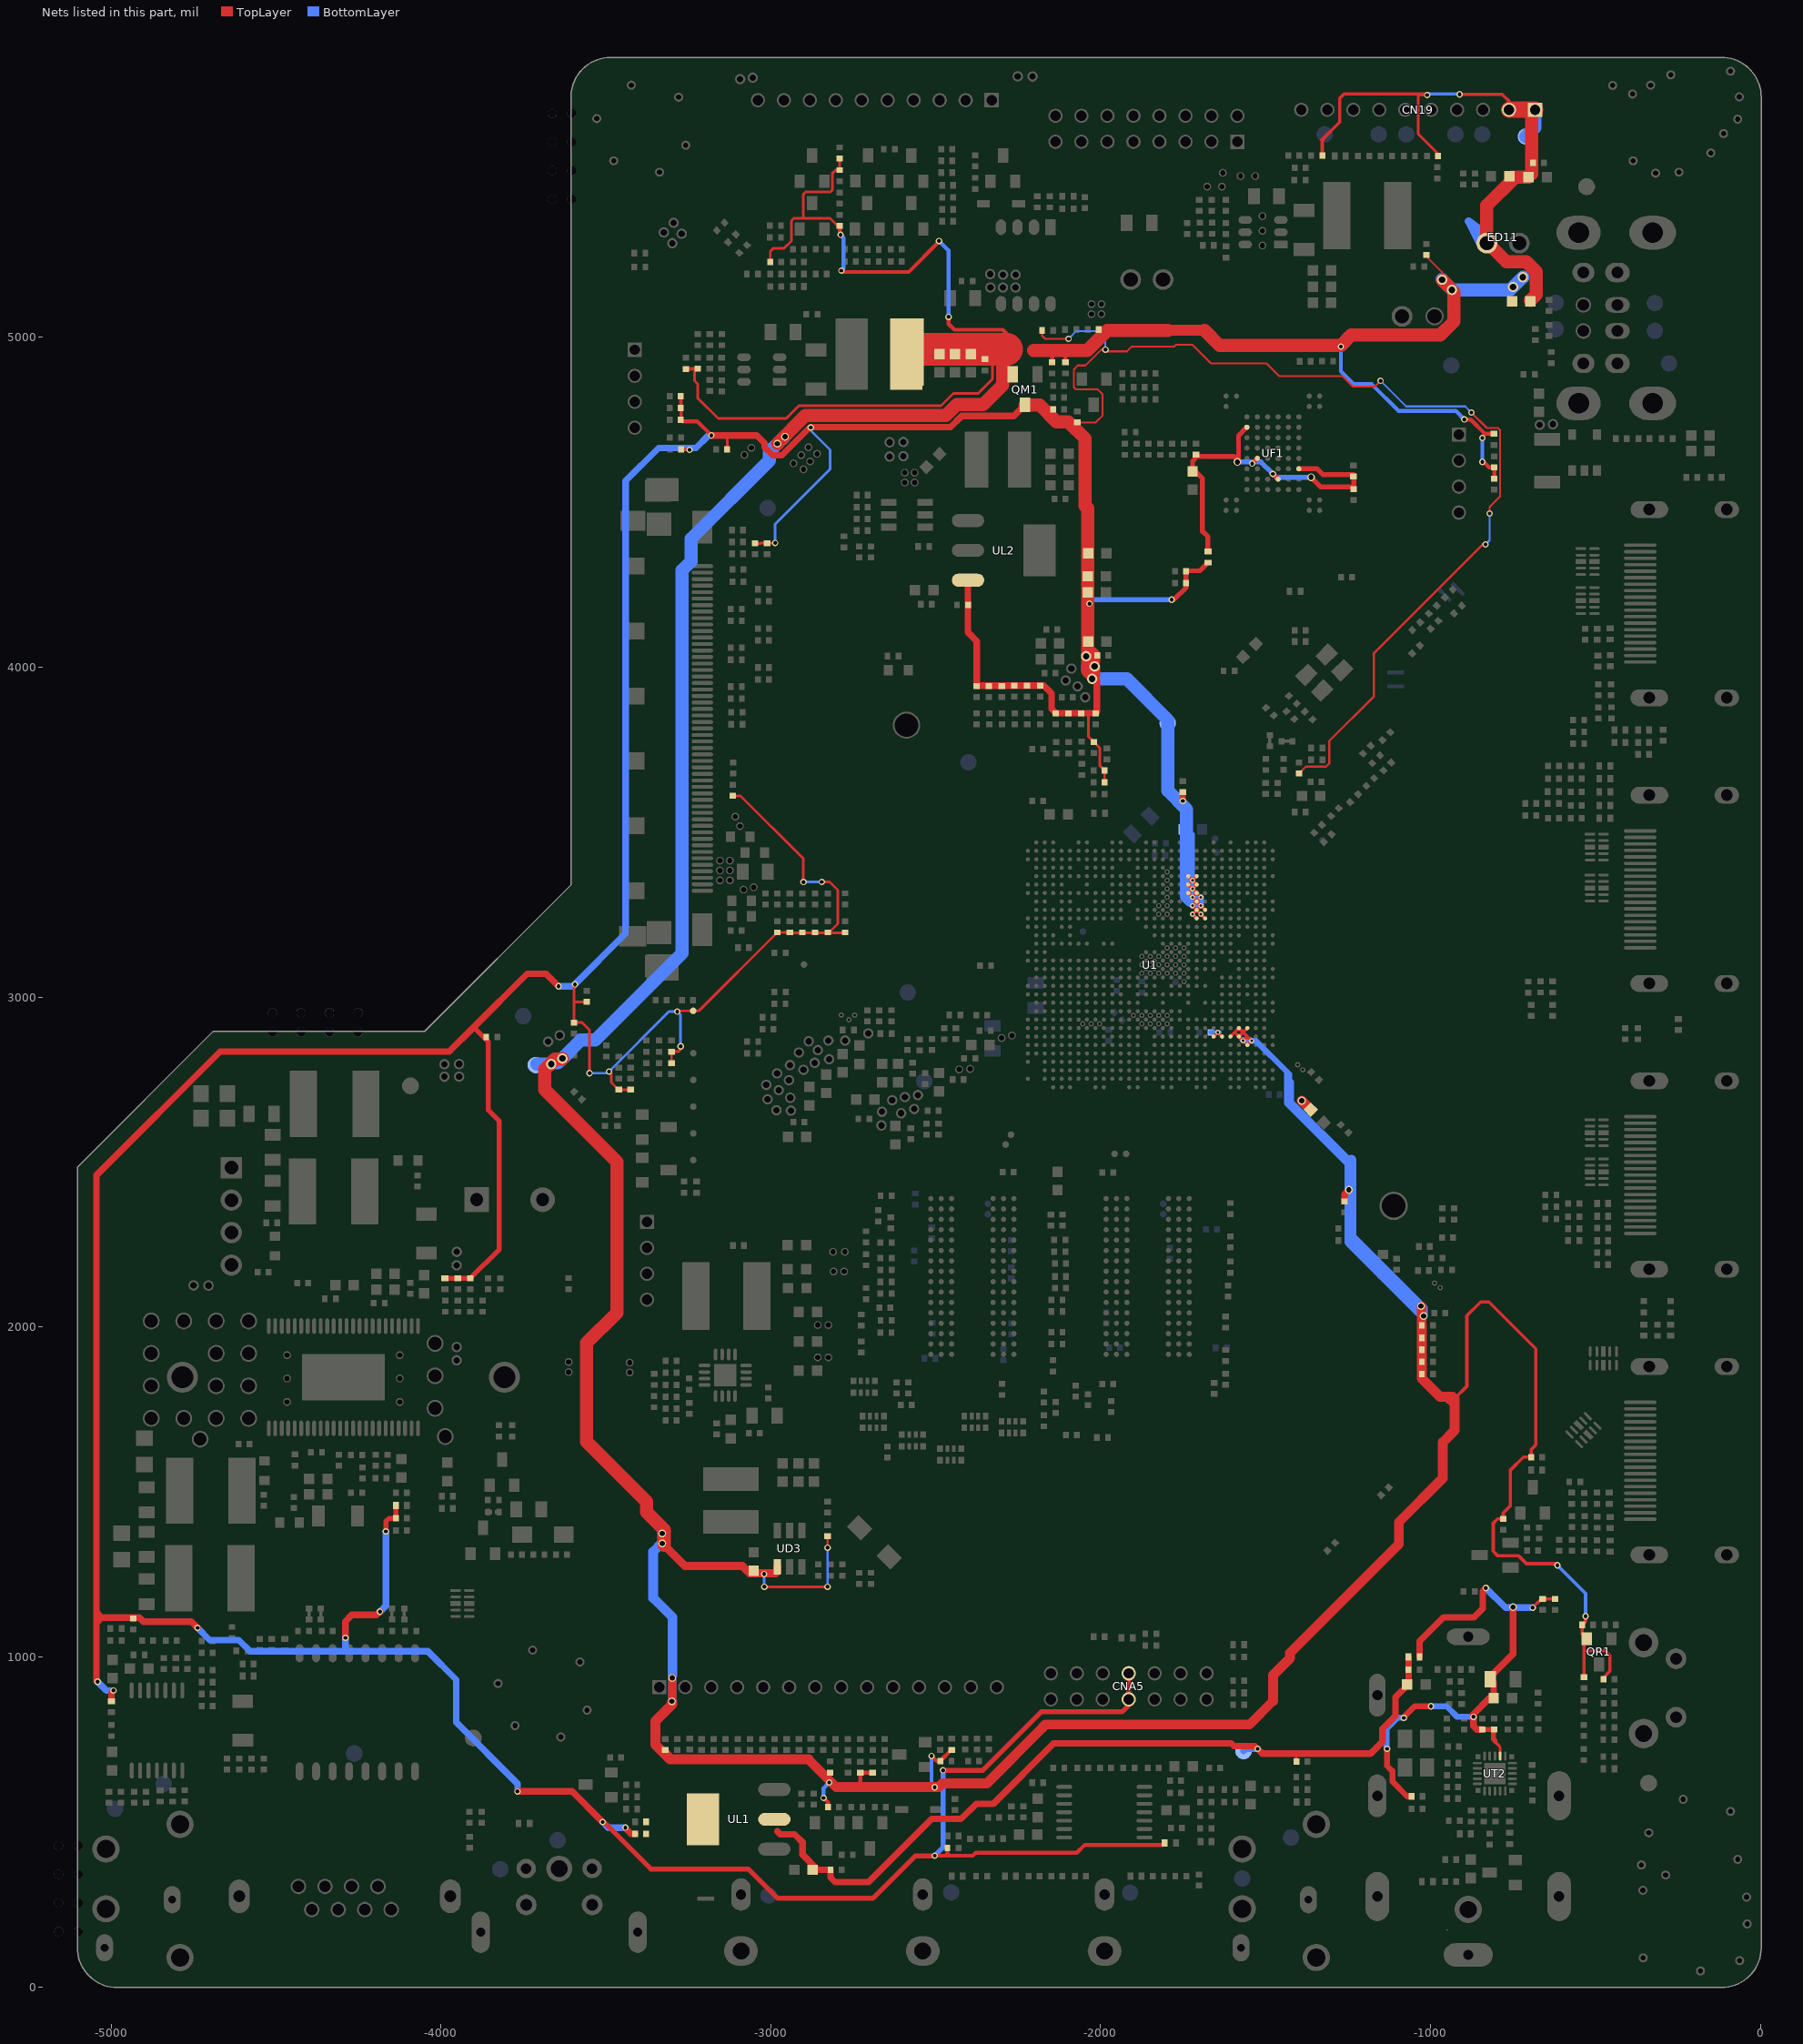
[diagram p0: the nets of this part, all layers, seen from the top]
# Altium PCB MISC86290.PcbDoc (part 9 of 31)
Units mil, origin at the board's own origin, x right, y up, seen from the top; angles counter-clockwise.
Board outline 5104.71 x 5851.49 mil, 2 copper layers (TopLayer, BottomLayer), stack 61.855 mil thick; 1026 components, 667 nets, 4280 pads, 2294 vias.

## Via types
v1: diameter 19.68, hole 11.81, TopLayer to BottomLayer, tented both sides, 1189 vias
v2: diameter 19.68/19.68 (per signal layer), hole 11.81, TopLayer to BottomLayer, tented both sides, 366 vias
v3: diameter 15.75, hole 7.87, TopLayer to BottomLayer, tented both sides, 348 vias
v4: diameter 23.62, hole 15.75, TopLayer to BottomLayer, tented both sides, 309 vias
v5: diameter 15.75/15.75 (per signal layer), hole 7.87, TopLayer to BottomLayer, tented both sides, 59 vias
v6: diameter 24/24 (per signal layer), hole 16, TopLayer to BottomLayer, tented both sides, 23 vias

## Nets (pads, with @x,y where several pads share a name; then routed paths per layer and width w, separated by ;. In a path a pad name is that pad's centre, name@x,y a point inside that pad or via, vN(x,y) a via of type N, cw(c..) or ccw(c..) an arc to the next point about the centre after c; other vN are vias at no path point) (continued)
3V3_M: 3V3_M.1 3V3_N.1 C16.2 C17.1 C18.1 C19.2 C20.1 C21.2 C22.1 C23.1 C240.2 CL55.2 CM2.2 CM3.2 CNA5.7 CNA5.8 LA10.1 LA12.1 LF1.2 LO2.2 LO3.2 pad.VIA5@-1696.18,3251.57 pad.VIA5@-1696.18,3277.17 pad.VIA5@-1696.18,3302.76 pad.VIA5@-1721.77,3251.57 pad.VIA5@-1721.77,3277.17 pad.VIA5@-1721.77,3302.76 pad.VIA5@-1721.77,3328.35 pad.VIA5@-1721.77,3353.94 pad.VIA5@-2018.5,4002.5 pad.VIA5@-2026,3965 pad.VIA5@-2044,4033.5 QM1.D R4.2 R5.2 R6.2 R7.2 R12.2 R13.2 R14.2 R15.2 R16.2 R17.2 R18.2 R19.2 R30.2 R31.2 R122.2 R124.2 R143.2 R144.2 R145.2 R171.2 R206.2 R207.2 RA5.1 RA34.1 RD24.2 RG6.2 RG16.2 RO46.2 RO47.2 RP5.2 RT7.2 RT40.1 RU5.1 RW8.1 RW9.1 RW251.2 RW405.2 RW406.2 RW407.2 RW408.2 RW409.2 RW410.2 U1.AA9 U1.AA10 U1.AB9 U1.AB10 U1.AC10 U1.AD10 U1.AD11 U1.AE10 U1.AE11 U1.AF10 U1.AF11 UL2.3 | length 23311.8
  TopLayer w6: RP5.2@-2177.73,5024 RP5.2@-2177.73,5021 -2177.73,5005.25 -2167.98,4995.5 v1(-2097.5,4995.5) ; C17.1@-2071,4742.27 -2015.22,4742.27 -1994,4763.49 -1994,4827.5 -2008.73,4842.23 -2075.45,4842.23 -2081.5,4848.28 -2081.5,4903 -2069.5,4915 -2046,4915 -1998,4963 v1(-1985.5,4963) -1980.16,4957.66 -1920.61,4957.66 -1905.61,4972.66 -1777.22,4972.66 -1771.89,4977.99 -1722.49,4977.99 -1665.49,4920.99 -1497.05,4920.99 -1458.55,4882.5 -1267.05,4882.5 -1235.68,4851.13 -1168.87,4851.13 v1(-1151.5,4868.5) ; v1(-876,4772) -829.5,4725.5 -795.5,4725.5 -789.16,4719.16 -789.16,4518.29 -821,4486.45 v1(-821,4466)
  TopLayer w7: RT7.2@-1398.5,3678.27 -1377.93,3698.84 -1316.66,3698.84 -1307.5,3708 -1307.5,3776.08 -1171.77,3911.81 -1171.77,4042.92 -842.22,4372.47 v1(-833.25,4372.47)
  TopLayer w8: -3596.97,2985.47 RG16.2@-3557.76,2985.47 ; v1(-3594.16,3038.7) -3597,3035.86 R143.2@-3597,2922.73 -3572.12,2922.73 -3549.35,2899.97 v1(-3549.35,2769.45) v1@-3549.35,2765.16 ; v1(-3490.5,2774.5) -3483.5,2767.5 -3483.5,2741 -3461.77,2719.27 R145.2@-3425,2719.27 ; R207.2@-3301,2800.23 R206.2@-3301,2834.77 -3280.23,2834.77 -3273.5,2841.5 v1(-3273.5,2851) ; v1(-3283.5,2956) -3284,2956.5 -3284,2958.5 3V3_N.1@-3235.5,2958.5 -3218.27,2958.5 RW405.2@-2980.5,3196.27 RW406.2@-2942.5,3196.27 ; R30.2@-3272.77,4750.37 R31.2@-3272.77,4786.37 ; RD24.2@-3272.27,4660.5 -3247.62,4660.5 v1(-3246.62,4659.5) ; R30.2@-3270.77,4754.26 R31.2@-3270.77,4786.37 ; RG6.2@-3132.5,4661 -3132.5,4700 ; RW408.2@-3115,3610.27 -3092.07,3610.27 -2902,3420.2 -2902,3348 v1(-2901,3349) ; RW8.1@-3047.5,4375.73 -3032,4375.73 -3030.83,4376.9 v1(-2986.82,4376.9) ; RW406.2@-2942.5,3194.8 RW409.2@-2824.55,3194.8 ; v1(-2879,4726.5) v1@-2877.5,4728 ; v1(-2845.66,3349.34) -2821.34,3349.34 -2796.75,3324.75 -2796.75,3222.6 RW409.2@-2824.55,3194.8 ; RW407.2@-2776.47,3194.8 RW409.2@-2824.55,3194.8 ; -2041.73,3860.73 -2037,3856 -2037,3789.73 R17.2@-2021,3773.73 -2002.16,3754.89 -2002.16,3727.68 -2003,3726.84 -2003,3701.73 R19.2@-1988.27,3687 R7.2@-1988.27,3651
  TopLayer w10: RW407.2@-2776.47,3194.8 RW407.2@-2775,3196.27 ; -2472.46,397 -2464.73,404.73 ; RO46.2@-2464.73,421 -2464.73,404.73 ; -2457,397 -2464.73,404.73 ; -2236.07,3943.23 R14.2@-2223.75,3943.23 ; U1.AF11@-1734.57,3366.73 pad.VIA5@-1721.77,3353.94 ; U1.AA10@-1708.98,3238.78 pad.VIA5@-1721.77,3251.57 U1.AB10@-1708.98,3264.37 ; U1.AF10@-1708.98,3366.73 pad.VIA5@-1721.77,3353.94 ; U1.AA9@-1683.39,3238.78 pad.VIA5@-1696.18,3251.57 U1.AB10@-1708.98,3264.37 ; U1.AB9@-1683.39,3264.37 pad.VIA5@-1696.18,3277.17 ; pad.VIA5@-1721.77,3302.76 U1.AC10@-1708.98,3289.96 ; pad.VIA5@-1721.77,3302.76 U1.AD11@-1734.57,3315.55 pad.VIA5@-1721.77,3328.35 ; pad.VIA5@-1721.77,3302.76 U1.AD10@-1708.98,3315.55 ; pad.VIA5@-1721.77,3328.35 U1.AE10@-1708.98,3341.14 pad.VIA5@-1721.77,3353.94 ; pad.VIA5@-1721.77,3328.35 U1.AE11@-1734.57,3341.14 pad.VIA5@-1721.77,3353.94 ; pad.VIA5@-1721.77,3328.35 U1.AD10@-1708.98,3315.55 ; U1.AB10@-1708.98,3264.37 pad.VIA5@-1696.18,3277.17 ; U1.AB10@-1708.98,3264.37 pad.VIA5@-1721.77,3277.17 U1.AC10@-1708.98,3289.96 ; U1.AC10@-1708.98,3289.96 pad.VIA5@-1696.18,3277.17 ; U1.AC10@-1708.98,3289.96 pad.VIA5@-1696.18,3302.76 U1.AD10@-1708.98,3315.55
  TopLayer w12: R31.2@-3272.77,4786.37 R171.2@-3272.77,4822.37 ; R30.2@-3267.74,4745.34 -3222.84,4745.34 v1(-3180.5,4703) ; v1(-2503.25,397) -2472.46,397 -2457,397 -2387.21,397 -2378.21,406 -2072.37,406 -2048.37,430 -1811.73,430 LO2.2@-1805.74,436
  TopLayer w15: v1(-4167,1380) -4167,1410 -4157,1420 RA5.1@-4136.73,1420 LA12.1@-4136.73,1459 ; LA10.1@-3988,2147.73 -3911,2147.73 -3823,2235.73 -3823,2623.97 -3856.4,2657.37 -3856.4,2864.4 -3901.01,2909.01 ; v1@-3509.73,502.73 -3364,357 -3068,357 -2979,268 -2690.79,268 -2561.79,397 v1(-2503.25,397) ; v1(-2478,656) -2357.51,656 -2180.01,833.5 -1935.5,833.5 -1915,854 CNA5.8@-1915,871.26 CNA5.7@-1915,950 CNA5.7@-1915,962 ; v1(-1785,4205) -1778.18,4205 -1741.27,4241.92 C22.1@-1741.27,4255 C23.1@-1741.27,4291 ; C23.1@-1733.87,4292.37 -1699.89,4292.37 LF1.2@-1675,4317.26
  TopLayer w17: v1(-1751,3594.5) C18.1@-1751,3621.27
  TopLayer w20: v1(-5041,924.5) -5044.17,927.67 -5044.17,1104 ; LO3.2@-4999,870 -4999,892 v1(-4993,898) ; v1(-4738,1088) -4756.5,1106.5 -4902.07,1106.5 -4914.57,1119 -5029.17,1119 ; v1(-4289.5,1057.5) -4289.5,1107.5 -4270,1127 -4195,1127 v1(-4185,1137) ; v1(-3768,592) -3602.38,592 v1@-3513.11,502.73 ; v1@-3643.6,3032.9 -3681.7,3071 -3739.02,3071 -3901.01,2909.01 -3975.12,2834.89 -4669.65,2834.89 -5044.17,2460.37 -5044.17,1134 ; v1(-3441,482.28) -3440.91,480.66 -3423.4,463.15 RT40.1@-3412,463.15 ; v1(-3180.5,4703) -3042.64,4703 -3019.25,4679.6 -3019.25,4667.75 -2994.13,4642.63 -2966.28,4642.63 -2880.92,4728 -2877.5,4728 -2455.26,4728 -2421.48,4761.78 -2263.22,4761.78 -2229.28,4795.72 QM1.D@-2229,4795.72 ; UL2.3@-2402.27,4263.87 -2402.27,4105.43 -2375.86,4079.02 -2375.86,3955.06 ; R13.2@-2374.86,3944.23 R12.2@-2261.75,3944.23 R14.2@-2223.75,3944.23 -2172.06,3944.23 -2148.9,3921.07 -2148.9,3873.64 R4.2@-2136,3860.73 ; R4.2@-2134.32,3862.41 -2132.64,3860.73 R5.2@-2098,3860.73 -2041.73,3860.73 RU5.1@-2015,3860.73 -2011.45,3864.28 pad.VIA5@-2011.45,3960.45 ; -5044.17,1104 -5029.17,1119 ; -5044.17,1104 -5044.17,1134 ; -5044.17,1134 -5029.17,1119
  TopLayer w40: QM1.D@-2229,4795.72 -2185.72,4795.72 -2134,4744 -2098,4744 -2046.84,4692.84 -2046.84,4488.84 -2039.83,4481.83 CM3.2@-2039.83,4275.9 -2039.83,4205.9 -2039.83,4055.06 ; pad.VIA5@-2021.45,4002.5 -2021.45,3975.55 -2024,3973 -2039.83,3988.83 -2039.83,4033.5 -2039.83,4055.06 ; -2021.45,4021.5 -2021.45,4035.5 -2021.45,4036.68 -2039.83,4055.06
  BottomLayer w6: v1(-2097.5,4995.5) -2073.5,5019.5 -2005,5019.5 -1985.84,5000.34 -1985.84,4963.34 v1(-1985.5,4963) ; v1(-1151.5,4868.5) -1074,4791 -895,4791 v1(-876,4772) ; v1(-833.25,4372.47) -821,4384.72 v1(-821,4466)
  BottomLayer w8: v1(-3594.16,3038.7) v1@-3591.96,3036.5 ; v1(-3549.35,2769.45) -3495.55,2769.45 v1(-3490.5,2774.5) -3309,2956 v1(-3283.5,2956) -3273.5,2946 v1(-3273.5,2851) ; v1(-3246.62,4659.5) v1@-3244,4659.5 ; v1@-2985.6,4376.9 v1(-2986.82,4376.9) -2986.82,4433.71 -2820,4600.53 -2820,4658.87 -2880.92,4719.79 -2880.92,4724.59 v1(-2879,4726.5) ; v1(-2901,3349) -2900.66,3349.34 v1(-2845.66,3349.34)
  BottomLayer w12: pad.VIA5@-1721.77,3328.35 -1703.31,3309.88 ; -1704.64,3308.55 -1703.31,3309.88 ; pad.VIA5@-1696.18,3302.76 -1703.31,3309.88
  BottomLayer w15: v1(-2503.25,397) -2477.91,422.34 v1@-2477.91,652.66 ; v1(-2034,4192.7) -2021.7,4205 -1985,4205 ; -2006,4205 -1985,4205 ; v1(-1785,4205) -1985,4205 ; pad.VIA5@-1722.02,3310.05 -1722.02,3494 ; pad.VIA5@-1721.77,3277.17 -1721.77,3287.58 pad.VIA5@-1721.77,3302.76 -1721.77,3308.55 -1708.22,3308.55 -1704.64,3308.55
  BottomLayer w18: pad.VIA5@-1721.77,3277.17 -1708.22,3277.17 ; -1708.22,3308.55 -1708.22,3277.17 ; pad.VIA5@-1696.18,3302.76 pad.VIA5@-1696.18,3277.17 -1708.22,3277.17
  BottomLayer w20: v1(-5041,924.5) -5014.5,898 v1(-4993,898) ; v1(-4738,1088) -4701,1051 -4612.67,1051 -4578.67,1017 -4040,1017 -3954,931 -3954,801.5 -3768,615.5 v1(-3768,592) ; -4289.5,1018 v1(-4289.5,1057.5) ; v1(-4185,1137) -4167,1155 v1(-4167,1380) ; v1(-3643.5,3033) -3600.08,3033 -3440.61,3192.47 -3440.61,3214.32 -3440.11,3214.82 -3440.11,4565.32 -3340.43,4665 -3227.25,4665 -3189.25,4703 v1(-3180.5,4703) ; v1(-3509.73,499.24) -3492.78,482.28 v1(-3441,482.28)
  BottomLayer w29.53: -1727.72,3293.53 -1721.77,3287.58
  BottomLayer w40: -2039.83,4002.5 -2039.83,3991.83 -2013,3965 -1921,3965 -1796,3840 -1796,3626 -1739.72,3569.72 -1739.72,3353.94 -1739.72,3305.53 -1727.72,3293.53
3V3_NAND: CF1.2 CF2.2 CF3.2 LF1.1 RF2.2 UF1.D3 UF1.G4 UF1.H8 UF1.J6 | length 1192.6
  TopLayer w15: CF3.2@-1721.5,4593.81 -1721.5,4625 -1707.23,4639.27 -1596.12,4639.27 -1582.19,4625.34 -1582.19,4702.18 UF1.D3@-1556.74,4727.63 ; CF3.2@-1718.25,4593.81 -1713.31,4593.81 -1691.75,4572.25 -1691.75,4412.27 -1675,4395.52 LF1.1@-1675,4350.73 ; v1@-1539.62,4618.76 UF1.G4@-1525.24,4633.14 ; v1@-1476.27,4585.26 -1462.25,4571.24 UF1.J6@-1462.25,4570.15 ; UF1.H8@-1399.26,4601.65 -1343.65,4601.65 -1326.54,4584.54 RF2.2@-1234,4584.54 ; v4(-1362.27,4576.26) -1332.74,4546.73 CF2.2@-1233.16,4546.73 ; RF2.2@-1233.16,4576.78 CF2.2@-1233.16,4546.73 ; CF2.2@-1233,4540.23 -1233.16,4540.23 CF2.2@-1233.16,4546.73
  BottomLayer w15: v4(-1585.27,4622.26) -1514.36,4622.26 v1(-1478,4585.9) -1468.36,4576.26 v4(-1362.27,4576.26)
  other v1: -1540.99,4617.39
3V3_STB: 3V3_STB.1 C12.2 C13.1 C14.1 C15.1 C27.1 C28.1 C29.1 CD15.2 CD16.2 CD17.2 CD18.2 CD19.2 CD21.2 CM4.2 LD2.1 LD3.2 LU11.1 pad.VIA5@-720.3,5182.7 pad.VIA5@-750,5153 pad.VIA5@-935,5144 pad.VIA5@-965,5175 pad.VIA5@-1021,2033.5 pad.VIA5@-1029,2063.5 pad.VIA5@-2957,4699 pad.VIA5@-2980.21,4678.2 pad.VIA5@-3298.97,936 pad.VIA5@-3300,865 pad.VIA5@-3329.25,1344 pad.VIA5@-3329.25,1374 pad.VIA5@-3631.84,2813.88 pad.VIA5@-3666,2797 QM1.S QR1.E R3.1 R137.2 R138.2 R139.2 R152.1 R153.1 RD15.1 RD21.2 RG7.2 RG17.2 RG30.2 RG38.2 RK1.2 RK13.2 RK23.1 RK24.2 RK34.2 RK42.2 RM2.1 RP1.2 RR2.2 RR3.2 RR9.2 RR13.2 RR17.2 U1.F4 U1.G5 U1.G6 U1.G7 U1.G8 U1.H4 U1.H5 UD3.4 | length 20811
  TopLayer w6: R152.1@-1013,5250.27 -1013,5246 -965,5198 pad.VIA5@-965,5175
  TopLayer w8: RD15.1@-3221.25,4905 -3221.71,4904.53 -3231.59,4894.66 -3231.59,4868.59 -3221.5,4858.5 -3221.5,4815.64 -3159.86,4754 -2953.7,4754 -2914.7,4793 -2483.85,4793 -2446.52,4830.33 -2371.49,4830.33 -2328,4873.82 -2328,4933 ; v1(-3019.5,1212.5) v1(-2828,1212.5) ; RG30.2@-3001.73,5229 -3001.73,5260.77 -2992,5270.5 -2959.95,5270.5 -2938,5292.45 -2938,5353.32 -2930.32,5361 -2820.34,5361 RG7.2@-2797.11,5337.77 ; -2901.31,5362.69 -2901.31,5434.19 -2894.5,5441 -2819.5,5441 -2813.07,5447.43 -2813.07,5498.18 -2804.02,5507.23 RG38.2@-2791,5507.23 RG17.2@-2791,5542.77 ; v1(-2828,1331) RD21.2@-2828,1365.27
  TopLayer w9.84: U1.G8@-1657.8,2880.51 v3(-1645,2893.31) U1.G7@-1632.2,2880.51
  TopLayer w10: CD15.2@-3257.25,4904.53 RD15.1@-3221.71,4904.53 ; RK23.1@-2485.73,684 RK13.2@-2451.5,718.27 RK13.2@-2451,718.27 ; U1.G6@-1606.61,2880.51 -1593.82,2893.31 ; U1.H4@-1555.43,2906.1 -1568.23,2893.31 ; -927.5,1782.5 -889.84,1820.16 -889.84,2034.16 -848.16,2075.84 -823.19,2075.84 -681.38,1934.03 -681.38,1642.53 -695.23,1628.68 RR17.2@-695.23,1605.5 -718.41,1605.5 -758.78,1565.13 -758.78,1456.45 -779.5,1435.73 RR2.2@-779.5,1418 -797.23,1418 -810,1405.23 -810,1320 -796,1306 -733,1306 -709.43,1282.43 -620.7,1282.43 v1(-615.85,1277.59) ; R153.1@-540.46,1100.54 R153.1@-540.46,1097 ; RR3.2@-535,938.73 -535,1046.5 QR1.E@-526.5,1055 -540.46,1068.96 R153.1@-540.46,1097 ; -533,1018 -470,1018 -456,1004 -456,957 -475.73,937.27 RR9.2@-475.73,932 ; v1(-530,1123) -530,1107.46 R153.1@-540.46,1097 ; -1593.82,2893.31 U1.H5@-1581.02,2906.1 -1568.23,2893.31 ; -1593.82,2893.31 U1.G5@-1581.02,2880.51 ; U1.G5@-1581.02,2880.51 -1568.23,2893.31 ; U1.G5@-1581.02,2880.51 v3(-1568.23,2867.72) ; v3(-1568.23,2867.72) -1555.43,2880.51 ; v3(-1568.23,2867.72) U1.F4@-1555.43,2854.92 v3(-1542.64,2867.72) -1555.43,2880.51 ; -1568.23,2893.31 -1555.43,2880.51
  TopLayer w12: v1(-2840,572.5) -2826.98,559.48 RR13.2@-2826.98,544.99 ; v1(-2823,619) v1@-2819.63,622.37 ; RG7.2@-2791,5337.77 -2791,5313.5 v1(-2788.5,5311) ; v1(-2786.39,5202.34) -2782.55,5198.5 -2581.91,5198.5 -2490,5290.41 v1(-2490,5292.5) ; -2728.5,605.84 RK1.2@-2728.5,648.77 RK42.2@-2691.5,648.77 ; v1(-2513,699.5) -2497.5,684 RK23.1@-2485.73,684 ; RK23.1@-2485.73,680.99 RK23.1@-2485.73,684 ; v1(-2461,5062.34) -2461,5040.75 -2443.41,5023.16 -2297.41,5023.16 -2284.97,5010.72 -2284.97,4964 ; RK13.2@-2451.5,718.27 -2452.26,718.27 -2485.73,684.79 RK23.1@-2485.73,684 ; CM4.2@-2147,4924.27 -2147,4956.25 -2143,4960.25 ; -2111,4960.25 -2107,4956.25 RM2.1@-2107,4924.27 ; v1(-897.38,4751.12) -878.12,4751.12 -834.73,4707.73 ; v1@-843.13,4626.73 v1@-838.9,4622.5 ; v1(-843,4622.5) v1@-838.9,4622.5 ; v1(-843,4695.32) -843,4699.46 -834.73,4707.73 ; R137.2@-808,4707.73 -834.73,4707.73 ; R138.2@-807,4571.73 R139.2@-807,4606.27 -822.67,4606.27 v1@-838.9,4622.5
  TopLayer w20: C13.1@-1260.72,2381.22 -1260.72,2402.7 v6(-1247.67,2415.76)
  TopLayer w25: pad.VIA5@-3326.25,1344 -3326.25,1341.25 -3322.84,1337.84 -3260.66,1275.66 -3086.66,1275.66 -3072.19,1261.19 CD21.2@-3052,1261.19 ; pad.VIA5@-3300,865 pad.VIA5@-3299.28,865.72 ; pad.VIA5@-3299.28,865 pad.VIA5@-3299.28,865.72 ; -3299.28,882 pad.VIA5@-3299.28,865.72 ; pad.VIA5@-3298.97,936 -3298.97,866.03 pad.VIA5@-3299.28,865.72 ; CD21.2@-3065,1254 -2985.25,1254 -2980.65,1258.6 UD3.4@-2980.65,1272.88
  TopLayer w28: -2167.89,794 -2166.89,795 -1548.82,795 -1477.5,866.32
  TopLayer w30: -3304.18,690.68 -3319.21,705.7 -3321.94,705.7 ; pad.VIA5@-3299.28,865 -3299.28,856.09 -3350.09,805.28 -3350.09,733.86 -3321.94,705.7 ; -3156.54,689.68 -3192.16,689.68 -3305.91,689.68 -3321.94,705.7 ; -3154.9,689.68 -3102.25,689.68 ; -3045.35,689.68 -3102.25,689.68 ; -3043.72,689.68 -3008.29,689.68 ; -2969.6,689.68 -2935.17,689.68 ; -2885.69,688.68 -2801.85,604.84 v1(-2503.5,604.84) -2491,604.84 -2479.84,616 -2476.07,616 ; -2885.69,689.68 -2935.17,689.68 ; -2479.34,616.5 -2344.74,616.5 -2176.12,785.12 -2176.12,785.77 -2167.89,794 ; -1477.5,866.32 -1477.5,944.64 -1426.66,995.48 -1426.66,1011.47 -1096.09,1342.04 -1096.09,1408.34 -963.28,1541.15 -963.28,1649.83 -931,1682.11 -931,1682.82 ; v4(-1390.49,2685.99) C12.2@-1363.17,2658.67 ; C28.1@-1027,1969.5 pad.VIA5@-1027,2062 ; C14.1@-1026.46,1857.84 -1026.46,1843.69 ; R3.1@-1026.46,2004.84 C28.1@-1026.46,1967 -1026.46,1843.69 ; -963.78,1623.5 -963.78,1650.04 -931,1682.82 ; -3102.25,689.68 -2935.17,689.68 ; -1026.46,1843.69 -971.2,1788.43 -948.95,1788.43 ; -948.95,1788.43 -927.5,1766.98 ; -948.95,1788.43 -933.43,1788.43 -927.5,1782.5 -927.5,1766.98 ; -931,1682.82 -927.5,1686.32 -927.5,1766.98
  TopLayer w32: -1797.1,5020.66 -1795.77,5021.99 -1685.88,5021.99 -1684.55,5020.66
  TopLayer w40: -3682.54,2718.13 -3683.25,2718.84 ; pad.VIA5@-3631.84,2813.88 -3633.72,2812 -3654.39,2812 -3685.5,2780.89 -3685.5,2722.5 ; pad.VIA5@-3322.84,1337.84 -3322.84,1385.57 -3376.43,1439.16 -3376.43,1470.16 -3558.5,1652.23 -3558.5,1951.53 -3466.75,2043.28 -3466.75,2500.92 -3683.25,2717.42 ; pad.VIA5@-2980.21,4678.2 -2895.41,4763 -2469.76,4763 -2435.98,4796.78 -2356.21,4796.78 -2297,4855.99 -2297,4951.97 -2284.97,4964 ; -2283.56,4965 -2278.06,4970.5 ; -2203.25,4960.25 -2143,4960.25 -2111,4960.25 -2040.35,4960.25 -1979.94,5020.66 -1797.1,5020.66 ; -1684.55,5020.66 -1640.39,4976.5 ; -1639.89,4976 -1271.71,4976 -1240.71,5007 -970.79,5007 -928.59,5049.2 -928.59,5137.68 pad.VIA5@-963.46,5172.55 ; -3685.5,2721.09 -3685.5,2722.5 ; -3685.5,2721.09 -3685.5,2719.68 -3683.25,2717.42 ; -3685.5,2721.09 -3683.25,2718.84 ; -3685.5,2722.5 -3683.25,2720.25 -3683.25,2718.84 ; -3683.25,2717.42 -3683.25,2718.84
  TopLayer w98.43: LD3.2@-2564.25,4958.21 -2558.46,4964 -2284.97,4964
  BottomLayer w8: v1@-3020.25,1209.89 v1(-3020.25,1251) ; v1(-2828,1212.5) v1(-2828,1331)
  BottomLayer w10: v1(-615.85,1277.59) -530,1191.74 v1(-530,1123)
  BottomLayer w12: v1(-2840,572.5) -2840,602 ; v1@-2826.45,615.8 -2840,602.25 -2840,602 ; v1(-2823,619) -2840,602 ; v1(-2788.5,5311) -2780.16,5302.66 -2780.16,5208.58 v1(-2786.39,5202.34) ; v1(-2513,699.5) -2513,614.34 v1(-2503.5,604.84) ; v1(-2490,5292.5) -2461,5263.5 v1(-2461,5062.34) ; C29.1@-1666.96,2893.31 v3(-1645,2893.31) v3@-1639.79,2893.31 ; v3(-1568.23,2867.72) -1571.19,2870.67 v3@-1566.94,2870.67 ; v1(-1272,4972) -1272,4897.35 -1232.78,4858.13 -1178.2,4858.13 -1097.07,4777 -923.26,4777 v1(-897.38,4751.12) ; v1(-843,4622.5) v1(-843,4695.32)
  BottomLayer w15: v3@-1571.19,2870.67 -1572.19,2871.67 v3@-1546.59,2871.67 ; v3(-1568.23,2867.72) v3(-1542.64,2867.72)
  BottomLayer w17.72: v3(-1542.64,2867.72) -1529.53,2867.72 -1435.13,2773.32 ; -1435.13,2749 -1435.13,2773.32 ; -1428.91,2740.51 -1428.91,2767.1 -1435.13,2773.32
  BottomLayer w25: pad.VIA5@-3299.28,865 -3299.28,884 ; -3299.25,884 pad.VIA5@-3299.25,935.72 ; -1425.5,2673.81 -1425.5,2676.54 ; -1247.67,2314 v6(-1247.67,2415.76) -1247.67,2495.98
  BottomLayer w30: pad.VIA5@-3329.25,1374 -3329.25,1346 -3356.25,1319 -3356.25,1178.43 -3298.22,1120.4 pad.VIA5@-3298.22,944.5 ; -1428.91,2740.51 -1428.91,2679.95 -1425.5,2676.54 -1245.67,2496.71 -1245.67,2278.67 ; -1239.77,2507.19 -1239.77,2274.8 -1240.78,2273.78 ; -1065.31,2077.69 -1049.61,2062 pad.VIA5@-1029,2062 ; pad.VIA5@-1022.91,2034.59 pad.VIA5@-1024,2035.68 ; -1245.67,2268.9 -1245.67,2257.35 pad.VIA5@-1024,2035.68 ; -1245.67,2268.9 -1245.67,2278.67 ; -1245.67,2268.9 -1240.78,2273.78 ; -1245.67,2278.67 -1240.78,2273.78 ; -1240.78,2273.78 -1029.75,2062.75 pad.VIA5@-1029,2062 ; pad.VIA5@-1029,2062 -1024,2057 pad.VIA5@-1024,2035.68
  BottomLayer w40: 3V3_STB.1@-3709.5,2797 pad.VIA5@-3666,2797 pad.VIA5@-3666.27,2800.73 ; -3242.25,4387.63 -3242.25,4320.7 -3268.61,4294.33 -3268.61,3133.95 -3533.05,2869.51 -3576.21,2869.51 pad.VIA5@-3635.73,2810 ; -3242.25,4389 -3004,4627.25 -3004,4654.41 pad.VIA5@-2980.21,4678.2 pad.VIA5@-2959.41,4699 ; pad.VIA5@-965,5175 pad.VIA5@-934.5,5144.5 ; pad.VIA5@-935,5144 -759,5144 pad.VIA5@-720.3,5182.7 ; pad.VIA5@-3666.27,2800.73 -3657,2810 pad.VIA5@-3635.73,2810 ; pad.VIA5@-3666.27,2800.73 -3645,2800.73 pad.VIA5@-3635.73,2810
3V3_TUN: 3V3_Tun.1 CL2.2 CL3.1 CT3.2 CT33.2 FT1.1 RO23.1 RO26.1 RT40.2 UL1.2 UL1.4 | length 2495.7
  TopLayer w8: RO26.1@-1406.73,682.5 -1406.73,706.77
  TopLayer w20: -2980.25,471 -2971.25,462 -2928,462 -2904,438 -2904,400.66 -2857.67,354.33 CL3.1@-2818.98,354.33 -2818.98,330.98 -2805,317 -2704,317 -2512.16,508.84 -2423.16,508.84 -2378,554 -2326.33,554 -2142.83,737.5 -1604,737.5 -1595.75,729.25 -1532.25,729.25 v1(-1524,721) -1510,707 -1181.3,707 -1145.5,742.8 -1145.5,782 -1106.42,821.08 -1106.42,877.58 -1066.73,917.27 FT1.1@-1066.73,1000
  BottomLayer w20: 3V3_Tun.1@-1567,714 -1560,721 v1(-1524,721)
3V3_TUN_IC: CT20.2 CT28.2 CT30.2 CT31.2 FT1.2 RT4.1 RT5.2 RT6.2 UT2.9 | length 1714.6
  TopLayer w7.8: -792.68,730.58 -789.15,727.04 UT2.9@-789.15,699.52
  TopLayer w10: -806.99,744.88 -792.68,730.58 ; v1(-690.5,1149) -663.61,1175.89 RT6.2@-660.5,1175.89 ; RT6.2@-663.15,1175.51 RT5.2@-622.5,1175.51
  TopLayer w15: CT31.2@-845.03,779.42 -809.03,779.42 -809.03,750.46 -805.22,746.65
  TopLayer w18: v1(-1132,721) -1132,669.66 -1114.92,652.58 -1114.92,620.92 -1071,577 RT4.1@-1057.73,577 ; v1(-1081,815) -1081.42,815 -1082.42,816 -1048.42,850 v2(-999,850)
  TopLayer w20: FT1.2@-1033.26,1000 -1033.26,1047.24 -960.5,1120 -868,1120 -841.5,1146.5 -841.5,1199.5 v2(-832.5,1208.5) ; CT31.2@-842.82,779.87 -859.46,779.87 -869.87,790.29 v2(-869.87,818) -869.87,826.2 -821.46,874.61 CT30.2@-808.63,874.61 -808.63,922.42 CT28.2@-818.82,932.61 ; CT28.2@-816,945 -813.5,945 -750,1008.5 v4(-750,1151)
  BottomLayer w18: v1(-1132,721) -1132.68,721.68 -1132.68,783.32 -1101,815 v1(-1081,815) ; v2(-999,850) -951,850 -919,818 v2(-869.87,818)
  BottomLayer w20: v2(-832.5,1208.5) -773,1149 v1(-690.5,1149)
3V3_WIFI: 3V3_WIFI.1 CN19.1 CN19.2 CU14.2 CU15.2 CU16.2 ED11.1 LU11.2 RU11.2 RU12.2 | length 1913.2
  TopLayer w8: -1037,5735 -1037,5616 -977.52,5556.52 RU12.2@-977.52,5550
  TopLayer w10: RU11.2@-1328.27,5551 -1328.27,5599.73 -1275,5653 -1275,5725 -1262,5738 -1013.27,5738 v1(-1010.27,5735) -1037,5735 ; v1(-912,5737) -783,5737 -761.97,5715.97 CN19.2@-761.97,5690.24
  TopLayer w40: CU15.2@-754.68,5486 CU16.2@-702.99,5486 ; CU15.2@-747.75,5481.45 -829.46,5399.75 -829.46,5288.87 -828.04,5287.44 -770.1,5229.5 -709.48,5229.5 -679.55,5199.58 -679.55,5130.13 LU11.2@-697.19,5112.5 ; CU16.2@-693.06,5495.93 -693.06,5680.41 CN19.1@-683.23,5690.24
  TopLayer w50: CN19.2@-761.97,5690.24 CN19.1@-683.23,5690.24
  BottomLayer w10: v1@-1007.27,5738 -913,5738 v1(-912,5737)
  BottomLayer w40: 3V3_WIFI.1@-711,5609 -683.23,5636.77 CN19.1@-683.23,5690.24